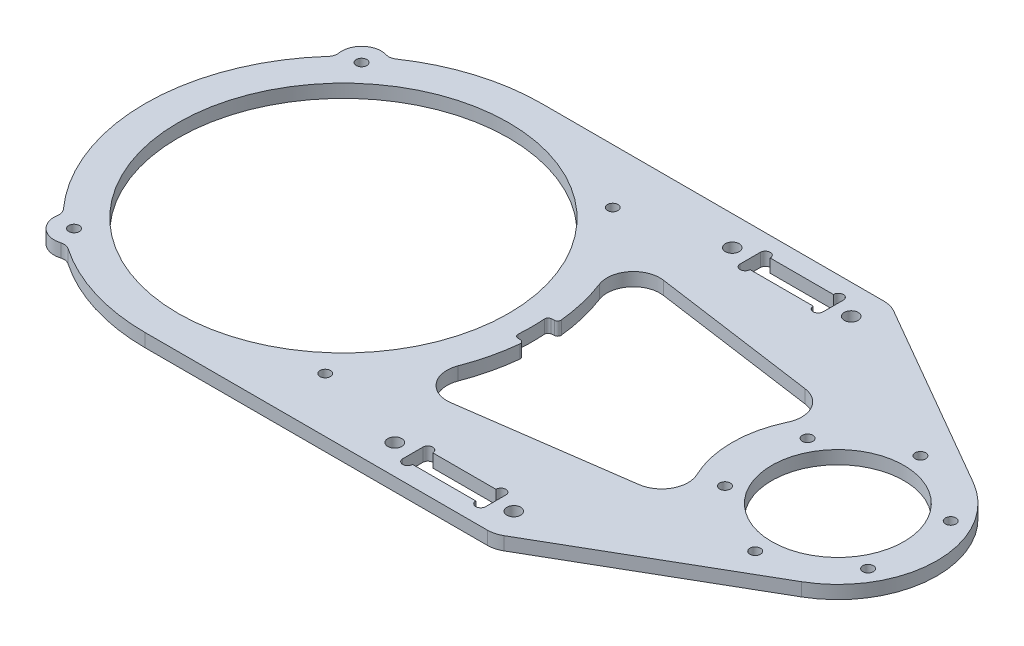
SolidWorks part; units mm, degrees
material "Thornel Mat VMA"
ref_plane "前视基准面" through (0, 0, 0) normal (0, 0, 1) x (1, 0, 0)
ref_plane "上视基准面" through (0, 0, 0) normal (0, 1, 0) x (1, 0, 0)
ref_plane "右视基准面" through (0, 0, 0) normal (1, 0, 0) x (0, 0, -1)
sketch "草图1" plane through (0, 0, 0) normal (0, 1, 0) x (1, 0, 0)
  line L0 (-84.5991, 0) -> (65, 0) construction
  line L1 (21.077, 60) -> (80, 25.9808)
  line L2 (21.077, -60) -> (80, -25.9808)
  line L5 (0, 0) -> (-64.7289, 35.8633) construction
  line L6 (-128.3348, 24.2319) -> (-40.8633, -24.2319) construction
  line L7 (-60.3671, 43.7357) -> (-108.831, -43.7357) construction
  line L8 (-84.5991, 50) -> (-84.5991, -50) construction
  line L9 (-18, 51.05) -> (18, 51.05) construction
  line L10 (-18, -51.05) -> (18, -51.05) construction
  line L11 (0, 51.05) -> (0, -51.05) construction
  line L12 (-9.55, 54.1) -> (9.55, 54.1)
  line L13 (-12.55, 54.1) -> (-12.55, 48)
  line L14 (-9.55, 48) -> (9.55, 48)
  line L15 (12.55, 54.1) -> (12.55, 48)
  line L16 (-9.55, -48) -> (9.55, -48)
  line L17 (-12.55, -54.1) -> (-12.55, -48)
  line L18 (-9.55, -54.1) -> (9.55, -54.1)
  line L19 (12.55, -54.1) -> (12.55, -48)
  line L22 (-84.5991, 60) -> (21.077, 60)
  line L23 (-84.5991, -60) -> (21.077, -60)
  line L24 (-35.3719, 34.3029) -> (43.0466, 23.2819)
  line L25 (43.0466, -23.2819) -> (-35.3719, -34.3029)
  line L26 (-27.816, 4.9679) -> (-24.8274, 5.2293)
  line L27 (-27.816, -4.9679) -> (-24.8274, -5.2293)
  circle A0 centre (-84.5991, 0) radius 50
  circle A1 centre (65, 0) radius 20
  arc A3 (80, -25.9808) -> (80, 25.9808) centre (65, 0) ccw
  circle A4 centre (65, 0) radius 25 construction
  circle A5 centre (65, 25) radius 1.6
  circle A6 centre (86.6506, 12.5) radius 1.6
  circle A7 centre (86.6506, -12.5) radius 1.6
  circle A8 centre (65, -25) radius 1.6
  circle A9 centre (43.3494, -12.5) radius 1.6
  circle A10 centre (43.3494, 12.5) radius 1.6
  circle A11 centre (-84.5991, 0) radius 41 construction
  circle A17 centre (-18, 51.05) radius 2.1
  circle A18 centre (18, 51.05) radius 2.1
  circle A19 centre (-18, -51.05) radius 2.1
  circle A20 centre (18, -51.05) radius 2.1
  arc A21 (-9.55, 54.1) -> (-12.55, 54.1) centre (-11.05, 54.1) ccw
  arc A22 (9.55, 54.1) -> (12.55, 54.1) centre (11.05, 54.1) cw
  arc A23 (9.55, 48) -> (12.55, 48) centre (11.05, 48) ccw
  arc A24 (-9.55, 48) -> (-12.55, 48) centre (-11.05, 48) cw
  arc A25 (-9.55, -48) -> (-12.55, -48) centre (-11.05, -48) ccw
  arc A26 (-9.55, -54.1) -> (-12.55, -54.1) centre (-11.05, -54.1) cw
  arc A27 (9.55, -54.1) -> (12.55, -54.1) centre (11.05, -54.1) ccw
  arc A28 (9.55, -48) -> (12.55, -48) centre (11.05, -48) cw
  arc A33 (-84.5991, 60) -> (-119.6283, 48.7129) centre (-84.5991, 0) ccw
  arc A37 (-35.3719, 34.3029) -> (-24.8274, 5.2293) centre (-84.5991, 0) cw
  arc A38 (43.0466, 23.2819) -> (43.0466, -23.2819) centre (65, 0) ccw
  arc A39 (-27.816, 4.9679) -> (-27.816, -4.9679) centre (-84.5991, 0) cw
  arc A40 (-24.8274, -5.2293) -> (-35.3719, -34.3029) centre (-84.5991, 0) cw
  circle A41 centre (-46.5991, 43.5) radius 1.6
  circle A42 centre (-122.5991, 43.5) radius 1.6
  circle A43 centre (-46.5991, -43.5) radius 1.6
  circle A44 centre (-122.5991, -43.5) radius 1.6
  arc A45 (-119.6283, 48.7129) -> (-128.1639, 41.2566) centre (-122.5991, 43.5) ccw
  arc A46 (-128.1639, 41.2566) -> (-128.1639, -41.2566) centre (-84.5991, 0) ccw
  arc A47 (-119.6283, -48.7129) -> (-128.1639, -41.2566) centre (-122.5991, -43.5) cw
  arc A48 (-119.6283, -48.7129) -> (-84.5991, -60) centre (-84.5991, 0) ccw
  point P27 (65, 0)
  point P49 (0, 51.05)
  dimension "D1" = 100
  dimension "D2" = 40
  dimension "D5" = 30
  dimension "D6" = 120
  dimension "D7" = 6
  dimension "D8" = 50
  dimension "D9" = 3.2
  dimension "D10" = 41
  dimension "D11" = 60
  dimension "D20" = 4.2
  dimension "D25" = 1.5
  dimension "D28" = 60
  dimension "D32" = 16
  dimension "D33" = 3
  dimension "D12" = 10
  dimension "D15" = 3.2
  dimension "D16" = 6
  dimension "D17" = 32
  dimension "D3" = 65
  dimension "D4" = 74
  dimension "D13" = 76
  dimension "D14" = 87
  dimension "D21" = 36
  dimension "D22" = 102.1
  dimension "D23" = 25.1
  dimension "D24" = 6.1
  dimension "D34" = 10
extrude "凸台-拉伸1" add sketch "草图1" along normal blind 4
fillet "R8 圆角1" radius 8 6 edges at (21.077, 2, -60) (21.077, 2, 60) (43.0466, 2, -23.2819) (43.0466, 2, 23.2819) (-35.3719, 2, -34.3029) (-35.3719, 2, 34.3029)
fillet "R2 圆角2" radius 1 4 edges at (-27.816, 2, -4.9679) (-24.8274, 2, -5.2293) (-27.816, 2, 4.9679) (-24.8274, 2, 5.2293)
fillet "R3 圆角" radius 3 4 edges at (-119.6283, 2, -48.7129) (-128.1639, 2, -41.2566) (-128.1639, 2, 41.2566) (-119.6283, 2, 48.7129)
